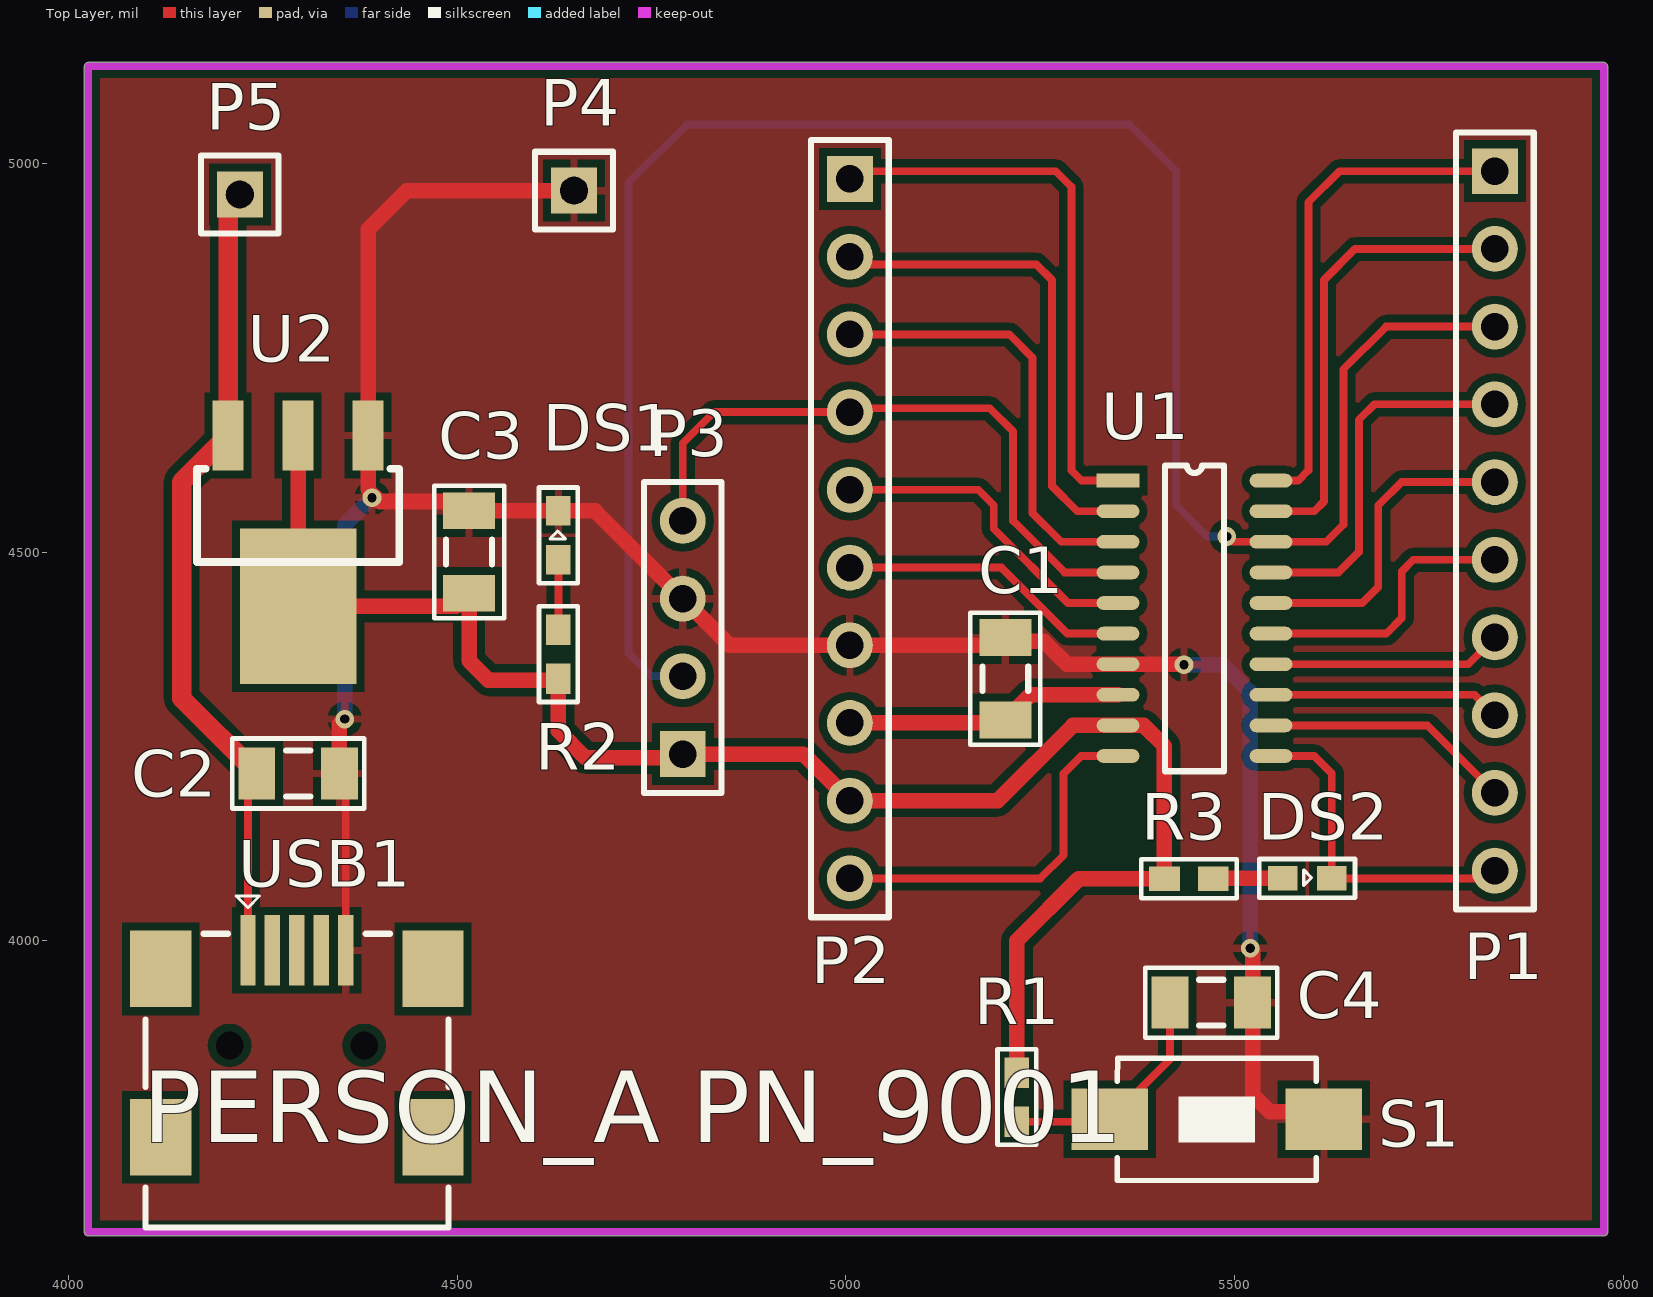
[diagram p0: Top Layer view]
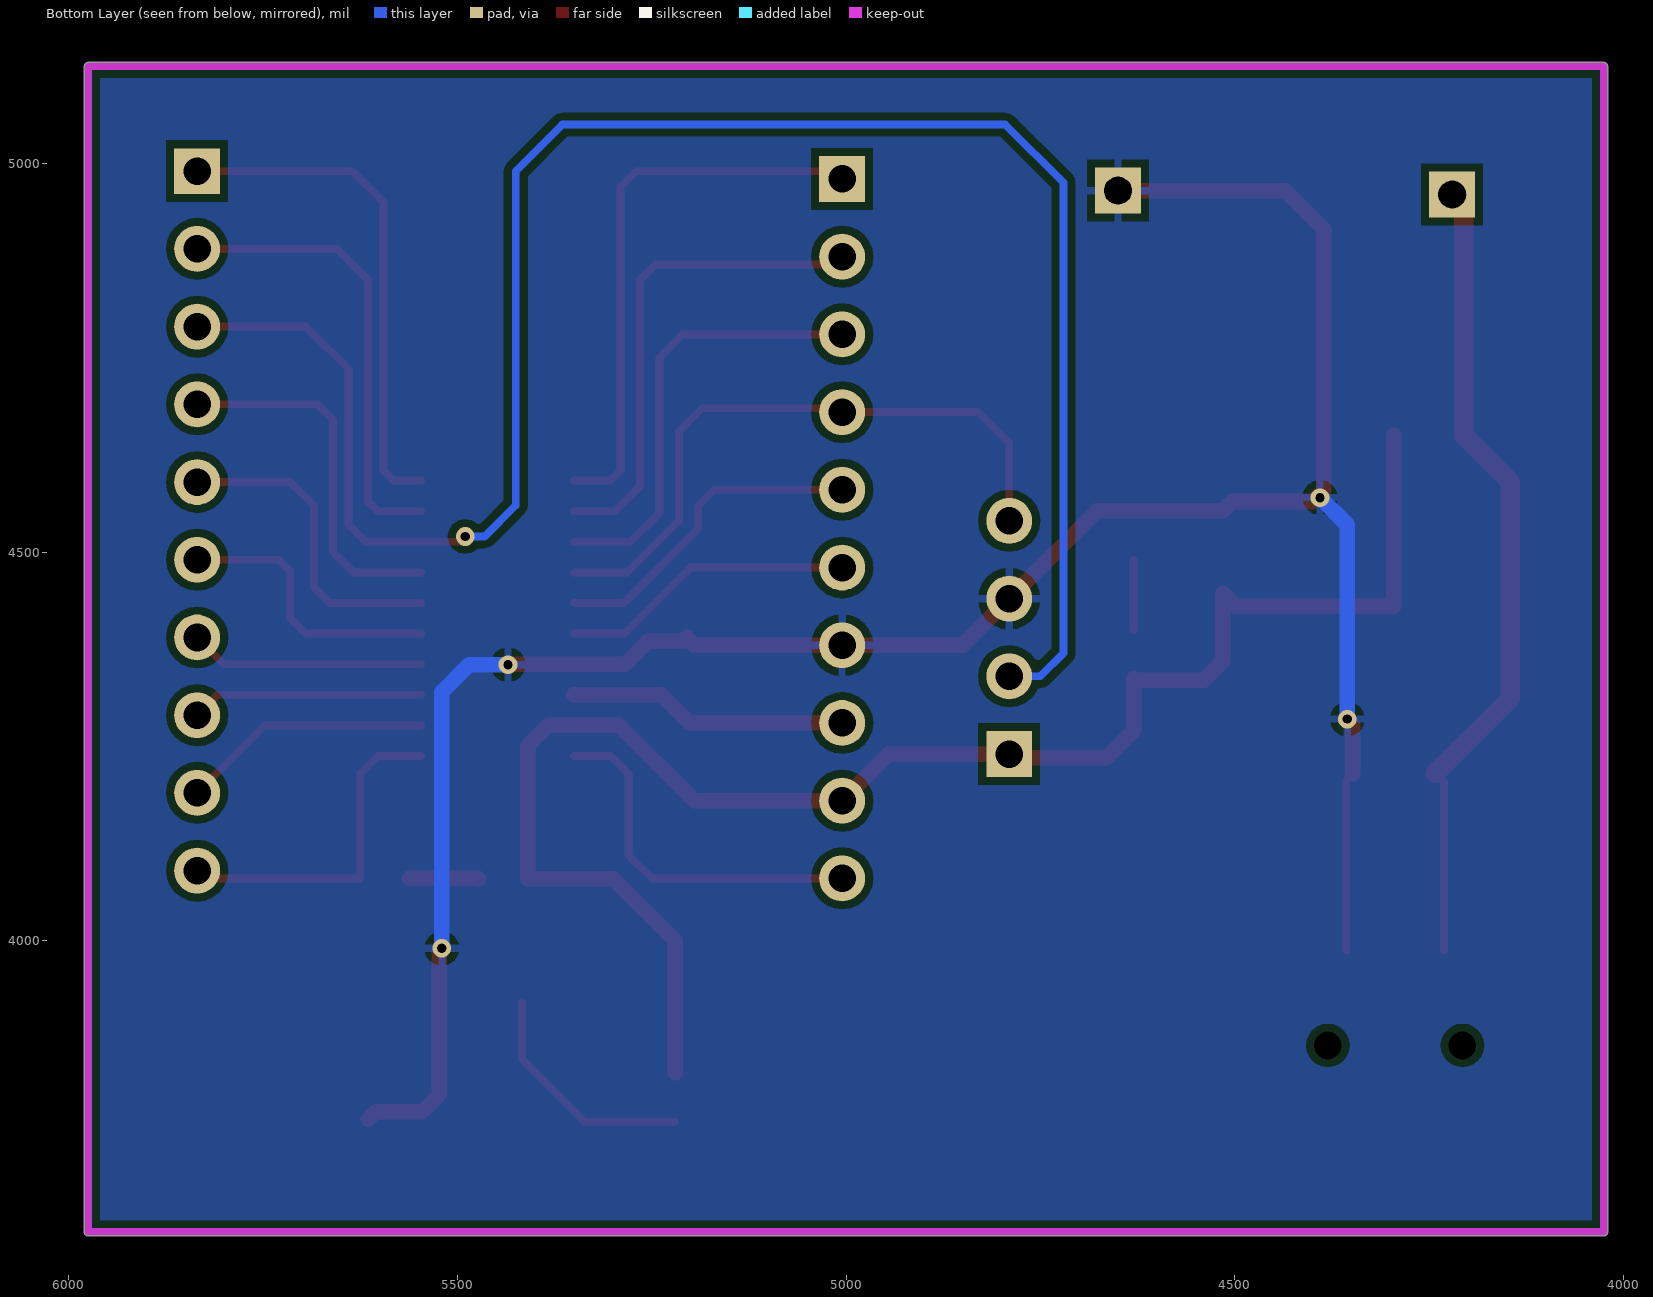
[diagram p1: Bottom Layer view, seen from below]
# Altium PCB MISC84379.PcbDoc
Units mil, origin at the board's own origin, x right, y up, seen from the top; angles counter-clockwise.
Board outline 1960.03 x 1510.03 mil, 2 copper layers (Top Layer, Bottom Layer); 18 components, 24 nets, 81 pads, 5 vias.

## Layer stack, top to bottom (the 12.6 mil dielectric is the usual default, probably not edited)
Top Solder: solder mask 0.4, Solder Resist, Dk 3.5
Top Layer: signal copper 1.4
Dielectric 1: dielectric 12.6, FR-4, Dk 4.8
Bottom Layer: signal copper 1.4
Bottom Solder: solder mask 0.4, Solder Resist, Dk 3.5

## Board outline
4019.99,3625 ccw(c4025,3625) 4025,3619.99 5975,3619.99 ccw(c5975,3625) 5980.02,3625 5980.02,5125 ccw(c5975,5125) 5975,5130.02 4025,5130.02 ccw(c4025,5125) 4019.99,5125

## Design rules (kind name [scope] priority, off if disabled: settings)
Clearance [All] p1: gap=10
MinimumSolderMaskSliver [All] p1: minsoldermaskwidth=0
PolygonConnect [All] p1: connectstyle=Relief reliefconductorwidth=10 reliefentries=4 polygonreliefangle="90 Angle" airgapwidth=10
RoutingVias [All] p1: holewidth=28 width=50 viastyle="Through Hole" minholewidth=28 minwidth=50 maxholewidth=28 maxwidth=50
SilkToSilkClearance [All] p1: silktosilkclearance=0
SilkToSolderMaskClearance [IsPad] p1: minsilkscreentomaskgap=0 clearancetoexposedcopper=TRUE
SolderMaskExpansion [All] p1: expansion=4
Width [All] p1: maxlimit=39.37 minlimit=10 preferedwidth=10
27 further rules are at their usual default settings.

## Components (designator, comment, footprint, x,y, rotation, side; value= is the part's Value field where it differs from the comment)
C1 "0.1UF" C1206 5205,4336.85 r270 top
C2 "0.1UF" C1206 4295,4215 r180 top
C3 "0.1UF" C1206 4515,4500 r270 top
C4 "0.1UF" C1206 5470,3920 r180 top
DS1 "LED2" my0603LED 4630,4490 r90 top
DS2 "LED2" my0603LED 5562.01,4080 r0 top
P1 "Header 10" HDR1X10 5835,4990 r270 top
P2 "Header 10" HDR1X10 5005,4980 r270 top
P3 "Header 4" HDR1X4 4790,4240 r90 top
P4 "HDR1X1" HDR1X1 4650,4965 r0 top
P5 "HDR1X1" HDR1X1 4220,4960 r0 top
R1 "Res2" my0603 5220,3767.01 r90 top
R2 "Res2" my0603 4630,4400 r270 top
R3 "Res2" my0603 5472.8,4079.53 r180 top
S1 "SW-PB" SW_PB2_A1 5475,3770 r270 top
U1 "STM8S103F3" SOP-20 5350,4591.85 r0 top
U2 "AMS1117" SOT223 4295,4650 r180 top
USB1 "MINI-USB" USB-MINI-A 4230.4,3987.36 r0 top

## Footprints (in the part's own frame and the unit in brackets; to place one, negate y for a bottom-side part, rotate by r counter-clockwise, add the part's x,y. Pads: shape width x height; smd on the part's side, far side on the other; paste and mask are expansions set on the pad)
C1206 [mm]
  rect 1.2x1.7 smd: 1(-1.35,0) 2(1.35,0)
  silkscreen extent -2.16,-1.14 2.16,1.14, body extent -1.7,-0.9 1.7,0.9, height 1.3
HDR1X1 [mm]
  rect 1.5x1.5 hole 0.9 slot 0.905 at 0 deg paste+0 mask+0.051: 1(0,0)
  silkscreen extent -1.27,-1.27 1.27,1.27
HDR1X4 [mm] "Connector; Header; 4 Position"
  rect 1.5x1.5 hole 0.9: 1(0,0)
  round 1.5 hole 0.9: 2(2.54,0) 3(5.08,0) 4(7.62,0)
  silkscreen extent -1.27,-1.27 8.89,1.27
HDR1X10 [mm] "Connector; Header; 10 Position"
  rect 1.5x1.5 hole 0.9: 1(0,0)
  round 1.5 hole 0.9: 2(2.54,0) 3(5.08,0) 4(7.62,0) 5(10.16,0) 6(12.7,0) 7(15.24,0) 8(17.78,0) 9(20.32,0) 10(22.86,0)
  silkscreen extent -1.27,-1.27 24.13,1.27
my0603 [mm]
  rect 1x0.8 smd: 1(0,0) 2(1.6,0)
  silkscreen extent -0.76,-0.64 2.36,0.64
my0603LED [mm]
  rect 0.965x0.8 smd: 1(0,0) 2(1.6,0)
  silkscreen extent -0.76,-0.64 2.36,0.64
SOP-20 [mm]
  rect 1.4x0.45 smd: 1(0,0)
  oval 1.4x0.45 smd: 2(0,-1) 3(0,-2) 4(0,-3) 5(0,-4) 6(0,-5) 7(0,-6) 8(0,-7) 9(0,-8) 10(0,-9) 11(5,-9) 12(5,-8) 13(5,-7) 14(5,-6) 15(5,-5) 16(5,-4) 17(5,-3) 18(5,-2) 19(5,-1) 20(5,0)
  silkscreen extent 1.53,-9.5 3.47,0.5
SOT223 [mil]
  rect 40x90 smd: 1(-90,0) 2(0,0) 3(90,0)
  rect 150x200 smd: 2(0,220)
  silkscreen extent -130,43 130,163, body extent -130,-30 126,246, height 65
SW_PB2_A1 [mm]
  rect 2x2.5 smd: 1(0,3.556) 2(0,-3.444)
  silkscreen extent -2,-3.19 2,3.31, body extent -2.03,-3.18 2.03,3.3, height 1.2
USB-MINI-A [mm]
  rect 2x2.5 smd: 0(-2.85,-6.108) 0(-2.85,-0.608) 0(6.05,-6.108) 0(6.05,-0.608)
  rect 0.5x2.3 smd: 1(0,0) 2(0.8,0) 3(1.6,0) 4(2.4,0) 5(3.2,0)
  round 0.6 hole 0.9 unplated: MH1(3.8,-3.108) MH2(-0.6,-3.108)
  silkscreen extent -3.35,-9.06 6.55,1.78, body extent -3.17,-9.04 6.33,0.66, height 3.95

## Part data
C1 C2 C3 C4: library part "Cap Semi", "Capacitor (Semiconductor SIM Model)"
DS1 DS2: "Typical RED, GREEN, YELLOW, AMBER GaAs LED"
P1 P2: "Header, 10-Pin"
P3: "Header, 4-Pin"
R1 R2 R3: "Resistor"
S1: "Switch"
U2: "Three-terminal regulator IC"

## Via types
v1: diameter 24, hole 12, Top Layer to Bottom Layer, 5 vias

## Nets (pads, with @x,y where several pads share a name; then routed paths per layer and width w, separated by ;. In a path a pad name is that pad's centre, name@x,y a point inside that pad or via, vN(x,y) a via of type N, cw(c..) or ccw(c..) an arc to the next point about the centre after c; other vN are vias at no path point)
3V3: C3.2 P2.9 P3.1 R1.2 R2.2 R3.2 U1.9 U2.2 | length 2162.9
  Top Layer w20: U2.2@4295,4650 4295,4430 4498.15,4430 C3.2 4515,4360 4540,4335 4627.99,4335 R2.2 4630,4270 4665,4235 4785,4235 P3.1 4945,4240 P2.9 5195,4180 5291.89,4276.89 U1.9 5383.11,4276.89 5409.8,4250.2 R3.2 5299.53,4079.53 5220,4000 R1.2
5V: C2.2 P5.1 U2.3 USB1.1 | length 1048.6
  Top Layer w10: USB1.1 4230.4,4203.55 C2.2
  Top Layer w25: P5.1 4205,4945 U2.3 4145,4590 4145,4311.85 C2.2
A1: P2.5 U1.5 | length 422.9
  Top Layer w10: P2.5 5170,4580 5190,4560 5190,4530 5285.63,4434.37 U1.5
A2: P2.6 U1.6 | length 380.2
  Top Layer w10: P2.6 5200,4480 5285,4395 U1.6
A3: P2.10 U1.10 | length 471.8
  Top Layer w10: P2.10 5250,4080 5280,4110 5280,4215 5302.52,4237.52 U1.10
B4: P1.9 U1.12 | length 324.1
  Top Layer w10: U1.12 5748.11,4276.89 P1.9
B5: DS2.2 P1.10 U1.11 | length 436.6
  Top Layer w10: U1.11 5602.48,4237.52 5625,4215 DS2.2 5825,4080 P1.10
C3: P1.8 U1.13 | length 299
  Top Layer w10: U1.13 5808.74,4316.26 P1.8
C4: P1.7 U1.14 | length 302.4
  Top Layer w10: U1.14 5800.63,4355.63 P1.7
C5: P1.6 U1.15 | length 362.6
  Top Layer w10: U1.15 5695,4395 5715,4415 5715,4475 5730,4490 P1.6
C6: P1.5 U1.16 | length 414.1
  Top Layer w10: U1.16 5664.37,4434.37 5685,4455 5685,4560 5715,4590 P1.5
C7: P1.4 U1.17 | length 477.3
  Top Layer w10: U1.17 5633.74,4473.74 5660,4500 5660,4670 5680,4690 P1.4
D1: P1.3 P3.2 U1.18 | length 2539.6
  Top Layer w10: v1(5490,4520) 5496.89,4513.11 U1.18 5618.11,4513.11 5640,4535 5640,4735 5695,4790 P1.3
  Bottom Layer w10: P3.2 4750,4340 4720,4370 4720,4975 4795,5050 5365,5050 5425,4990 5425,4560 5465,4520 v1(5490,4520)
D2: P1.2 U1.19 | length 594.9
  Top Layer w10: U1.19 5602.48,4552.48 5615,4565 5615,4850 5655,4890 P1.2
D3: P1.1 U1.20 | length 655.2
  Top Layer w10: U1.20 5581.85,4591.85 5595,4605 5595,4950 5635,4990 P1.1
D4: P2.1 U1.1 | length 727.9
  Top Layer w10: P2.1 5015,4990 5270,4990 5290,4970 5290,4605 5303.15,4591.85 U1.1
D5: P2.2 U1.2 | length 635.9
  Top Layer w10: P2.2 5015,4870 5245,4870 5265,4850 5265,4585 5297.52,4552.48 U1.2
D6: P2.3 U1.3 | length 572.7
  Top Layer w10: P2.3 5210,4780 5240,4750 5240,4550 5276.89,4513.11 U1.3
GND: C1.1 C2.1 C3.1 C4.1 DS1.2 P2.7 P3.3 P4.1 S1.1 U1.7 U2.1 USB1.5 | length 3099.6
  Top Layer w10: C2.1 4356.38,4206.77 USB1.5
  Top Layer w20: C2.1 4348.15,4278.15 v1(4355,4285) ; P4.1 4435,4965 4385,4915 U2.1 4385,4580 4400,4565 4503.15,4565 C3.1 4629.84,4553.15 DS1.2 4677.01,4552.99 P3.3 4850,4380 P2.7 5195,4380 C1.1 5210,4385 5255,4385 5284.37,4355.63 U1.7 5434.37,4355.63 v1(5435,4355) ; v1(5520,3990) 5523.15,3986.85 C4.1 5523.15,3801.85 5545,3780 5605,3780 S1.1
  Bottom Layer w20: v1(4355,4285) 4355,4535 v1(4390,4570) ; v1(5435,4355) 5485,4355 5520,4320 v1(5520,3990)
NetC4_2: C4.2 R1.1 S1.2 | length 302.7
  Top Layer w10: R1.1 5336.42,3767.01 S1.2 5416.85,3847.44 C4.2
NetDS1_1: DS1.1 R2.1 | length 90
  Top Layer w10: R2.1 DS1.1
NetDS2_1: DS2.1 R3.1 | length 89.4
  Top Layer w20: R3.1 5473.27,4080 DS2.1
NRST: P2.4 P3.4 U1.4 | length 833.5
  Top Layer w10: P3.4 4790,4640 4830,4680 P2.4 5010,4685 5185,4685 5215,4655 5215,4540 5281.26,4473.74 U1.4
VCAP: C1.2 P2.8 U1.8 | length 360
  Top Layer w20: P2.8 5201.3,4280 C1.2 5237.56,4316.26 U1.8
pads on no net: USB1.0 USB1.2 USB1.3 USB1.4 USB1.MH1 USB1.MH2

## Polygon pours and split planes (outlines as drawn)
GND on Bottom Layer "D" (solid, remove dead copper, pour order 0): 3925,5250 3950,5275 6105,5275 6105,3480 6195,3390 6030,3555 3970,3555
GND on Top Layer "D" (solid, remove dead copper, pour order 2): 3770,5345 6305,5345 6350,5300 6165,5115 6165,3365 3800,3365 3790,3375

## Keep-outs
Keep-Out Layer:
  lines w10: 4100,3625 5975,3625 5975,5125 4100,5125 4025,5125 4025,3625 4110,3625

## Silkscreen, mask and mechanical layers (free items; w line width, h text height)
Top Overlay:
  text "PERSON_A PN_9001" at 4095,3710 h157.48